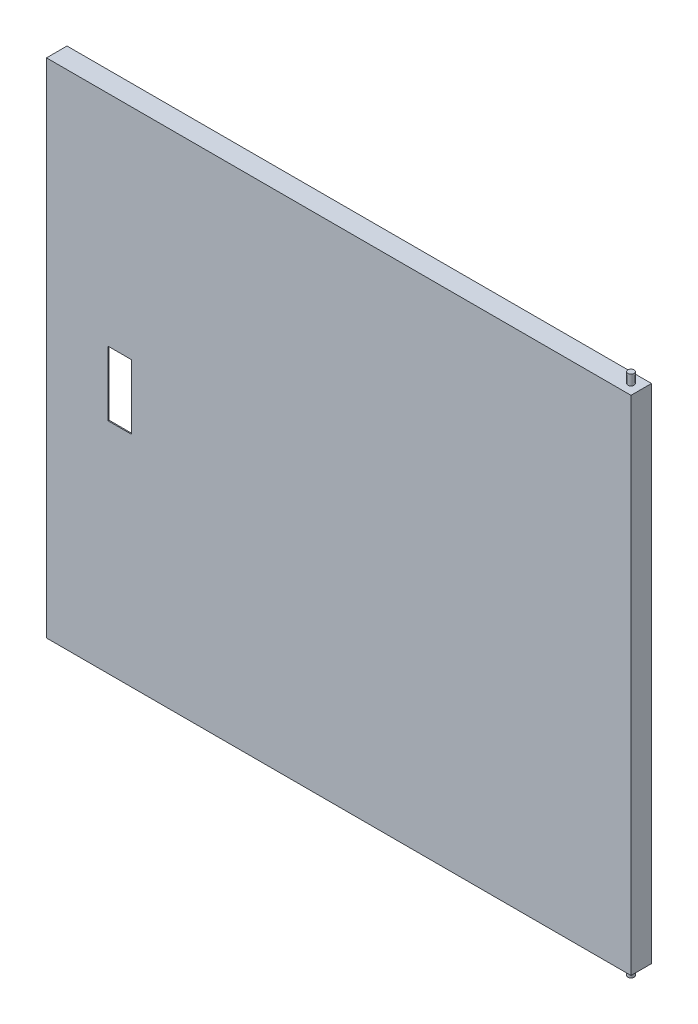
from build123d import *

# Parameters (mm, degrees)
SKETCH_1_W          = 570
SKETCH_1_H          = 490
EXTRUDE_1_DEPTH     = 20
SHELL_3_T           = -1
SKETCH_5_W          = 570
SKETCH_5_H          = 490
SKETCH_5_W_2        = 550
SKETCH_5_H_2        = 470
EXTRUDE_3_DEPTH     = 1.5
SKETCH_11_R         = 3
EXTRUDE_4_DEPTH     = 10
EXTRUDE_START       = 10
SKETCH_12_R         = 3
EXTRUDE_5_DEPTH     = 10
SKETCH_13_W         = 23
SKETCH_13_H         = 63
CUT_EXTRUDE_3_DEPTH = 1.5


with BuildPart() as part:
    # 草图1 → 凸台-拉伸1 (new body)
    with BuildSketch(Plane.XY):
        Rectangle(SKETCH_1_W, SKETCH_1_H)
    extrude(amount=EXTRUDE_1_DEPTH)

    # 抽壳3
    shell_3_openings = [part.faces().sort_by_distance(p)[0] for p in [
        (0, 0, 0),
    ]]
    offset(amount=SHELL_3_T, openings=shell_3_openings, kind=Kind.INTERSECTION)

    # 草图5 → 凸台-拉伸3 (add)
    with BuildSketch(Plane(origin=(0, 0, 0), x_dir=(-1, 0, 0), z_dir=(0, 0, -1))):
        Rectangle(SKETCH_5_W, SKETCH_5_H)
        Rectangle(SKETCH_5_W_2, SKETCH_5_H_2, mode=Mode.SUBTRACT)
    extrude(amount=-EXTRUDE_3_DEPTH)

    # 草图11 → 凸台-拉伸4 (add)
    with BuildSketch(Plane(origin=(0, 245, 0), x_dir=(1, 0, 0), z_dir=(0, 1, 0))):
        with Locations(Location((275, -10, 0), (0, 0, 90))):
            Circle(SKETCH_11_R)
    extrude(amount=EXTRUDE_4_DEPTH)

    # 草图12 → 凸台-拉伸5 (add)
    with BuildSketch(Plane.XZ.offset(245).offset(EXTRUDE_START)):
        with Locations(Location((275, 10, 0), (0, 0, 270))):
            Circle(SKETCH_12_R)
    extrude(amount=-EXTRUDE_5_DEPTH)

    # 草图13 → 切除-拉伸3 (cut)
    with BuildSketch(Plane.XY.offset(20)):
        with Locations((-213.5, 0)):
            Rectangle(SKETCH_13_W, SKETCH_13_H)
    extrude(amount=-CUT_EXTRUDE_3_DEPTH, mode=Mode.SUBTRACT)


solid = part.part
